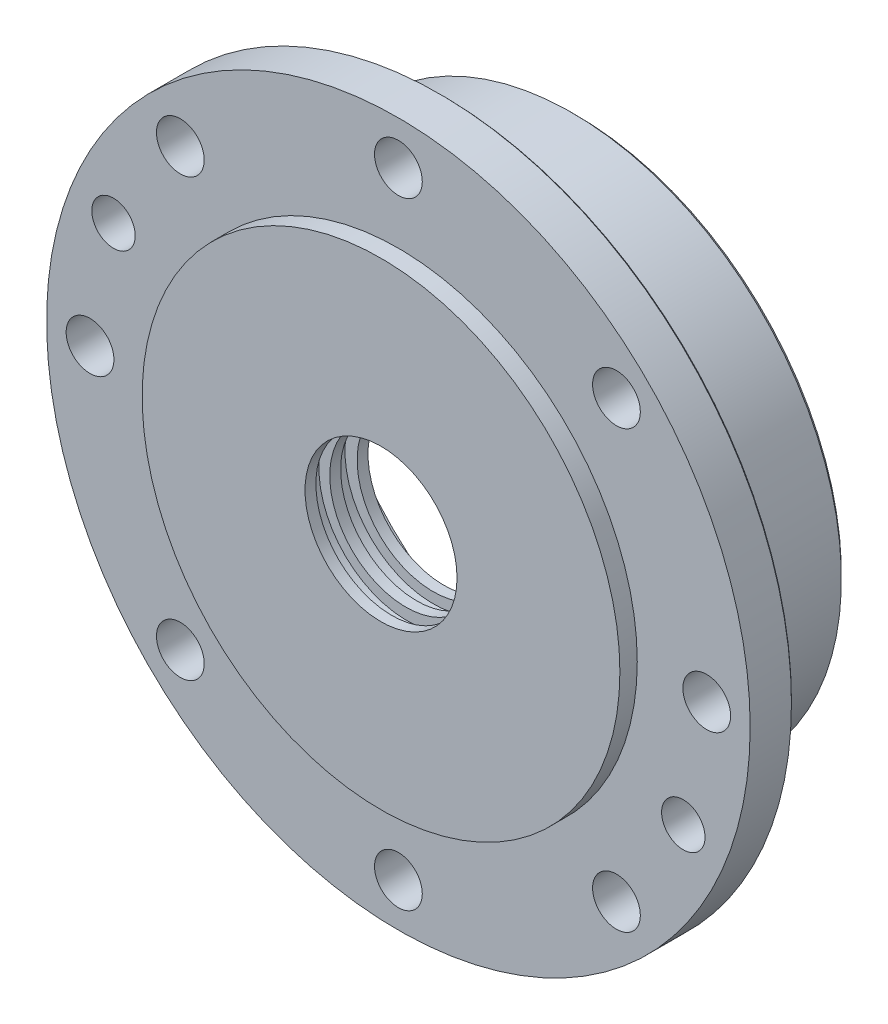
SolidWorks part; units mm, degrees
ref_plane "Front Plane" through (0, 0, 0) normal (0, 0, 1) x (1, 0, 0)
ref_plane "Top Plane" through (0, 0, 0) normal (0, 1, 0) x (1, 0, 0)
ref_plane "Right Plane" through (0, 0, 0) normal (1, 0, 0) x (0, 0, -1)
other "Configuration Table"
sketch "Sketch1" plane through (0, 0, 0) normal (0, 0, 1) x (1, 0, 0)
  circle A0 centre (0, 0) radius 81
  dimension "D1" = 162
extrude "Boss-Extrude1" add sketch "Sketch1" along normal blind 10
sketch "Sketch2" plane through (0, 0, 10) normal (0, 0, 1) x (1, 0, 0)
  circle A0 centre (0, 0) radius 55
  dimension "D1" = 110
extrude "Boss-Extrude2" add sketch "Sketch2" along normal blind 4
sketch "Sketch3" plane through (0, 0, 0) normal (0, 0, -1) x (-1, 0, 0)
  circle A0 centre (0, 0) radius 62
  dimension "D1" = 124
extrude "Boss-Extrude3" add sketch "Sketch3" along normal blind 31
sketch "Sketch4" plane through (0, 0, 14) normal (0, 0, 1) x (1, 0, 0)
  circle A0 centre (0, 0) radius 17.5
  dimension "D1" = 35
extrude "Cut-Extrude1" cut sketch "Sketch4" against normal blind 2.5
sketch "Sketch5" plane through (0, 0, 11.5) normal (0, 0, 1) x (1, 0, 0)
  circle A0 centre (0, 0) radius 20.3
  dimension "D1" = 40.6
extrude "Cut-Extrude2" cut sketch "Sketch5" against normal blind 3.5
sketch "Sketch6" plane through (0, 0, 8) normal (0, 0, 1) x (1, 0, 0)
  circle A0 centre (-0.3036, -0.2277) radius 17.5
  dimension "D1" = 35
extrude "Cut-Extrude3" cut sketch "Sketch6" against normal blind 2.5
sketch "Sketch7" plane through (0, 0, 5.5) normal (0, 0, 1) x (1, 0, 0)
  circle A0 centre (0, 0.3795) radius 20.3
  dimension "D1" = 40.6
extrude "Cut-Extrude4" cut sketch "Sketch7" against normal blind 3.5
sketch "Sketch8" plane through (0, 0, 2) normal (0, 0, 1) x (1, 0, 0)
  circle A0 centre (0, 0) radius 17.5
  dimension "D1" = 35
extrude "Cut-Extrude5" cut sketch "Sketch8" against normal blind 2.5
sketch "Sketch9" plane through (0, 0, -0.5) normal (0, 0, 1) x (1, 0, 0)
  circle A0 centre (0, 0) radius 50
  dimension "D1" = 100
extrude "Cut-Extrude6" cut sketch "Sketch9" against normal blind 1.5
sketch "Sketch14" plane through (0, 0, 10) normal (0, 0, 1) x (1, 0, 0)
  line L0 (0, 0) -> (0, 71) construction
  point P1 (0, 71)
  point P7 (0, 71)
  dimension "D1" = 71
hole_wizard "Ø1.0mm Blind Dowel Hole1" positions "Sketch14" profile "Sketch15" hole size "Ø1.0" standard "GB" end condition through all
sketch "Sketch15" plane through (0, 71, 10) normal (1, 0, 0) x (0, -1, 0)
  line L0 (0, 0) -> (0, 41)
  line L1 (0, 41) -> (5.5, 41)
  line L2 (5.5, 41) -> (5.5, 0)
  line L5 (5.5, 0) -> (0, 0)
  line L11 (0, -6.35) -> (0, 107.95) construction
  dimension "通孔孔直径" = 11
  dimension "通孔孔深度" = 41
pattern_circular "CirPattern1" count 8 over 360 about axis through (0, 0, 0) along (0, 0, 1) of "Ø1.0mm Blind Dowel Hole1"
sketch "Sketch16" plane through (0, 0, 10) normal (0, 0, 1) x (1, 0, 0)
  line L0 (-71, 0) -> (71, 0) construction
  line L1 (0, 0) -> (-65.5954, 27.1705) construction
  line L2 (0, 0) -> (65.5954, -27.1705) construction
  circle A0 centre (0, 0) radius 71
  point P7 (65.5954, -27.1705)
  point P8 (-65.5954, 27.1705)
  point P10 (-65.5954, 27.1705)
  point P12 (-65.5954, 27.1705)
  point P16 (65.5954, -27.1705)
  dimension "D1" = 22.5
  dimension "D2" = 22.5
hole_wizard "Ø10.0mm Blind Dowel Hole1" positions "Sketch16" profile "Sketch17" hole size "Ø10.0" standard "GB" end condition through all
sketch "Sketch17" plane through (65.5954, -27.1705, 10) normal (1, 0, 0) x (0, -1, 0)
  line L0 (0, 0) -> (0, 41)
  line L1 (0, 41) -> (5, 41)
  line L2 (5, 41) -> (5, 0)
  line L5 (5, 0) -> (0, 0)
  line L11 (0, -6.35) -> (0, 107.95) construction
  dimension "通孔孔直径" = 10
  dimension "通孔孔深度" = 41
sketch "Sketch18" plane through (0, 0, -2) normal (0, 0, 1) x (1, 0, 0)
  circle A0 centre (0, 0) radius 58
  dimension "D1" = 116
extrude "Cut-Extrude7" cut sketch "Sketch18" against normal blind 4
sketch "Sketch19" plane through (0, 0, -31) normal (0, 0, -1) x (-1, 0, 0)
  circle A0 centre (0, 0) radius 60
  dimension "D1" = 120
extrude "Cut-Extrude8" cut sketch "Sketch19" against normal blind 9 contours A0
sketch "Sketch20" plane through (0, 0, -22) normal (0, 0, -1) x (-1, 0, 0)
  circle A0 centre (0, 0) radius 60.5
  dimension "D1" = 121
extrude "Cut-Extrude9" cut sketch "Sketch20" against normal blind 3
sketch "Sketch21" plane through (0, 0, -19) normal (0, 0, -1) x (-1, 0, 0)
  circle A0 centre (0, 0) radius 57.5
  dimension "D1" = 115
extrude "Cut-Extrude10" cut sketch "Sketch21" against normal up to next
chamfer "Chamfer1" distance 1 angle 45 1 edges at (-62, 0, -31)
chamfer "Chamfer2" distance 0.5 angle 45 1 edges at (81, 0, 0)
